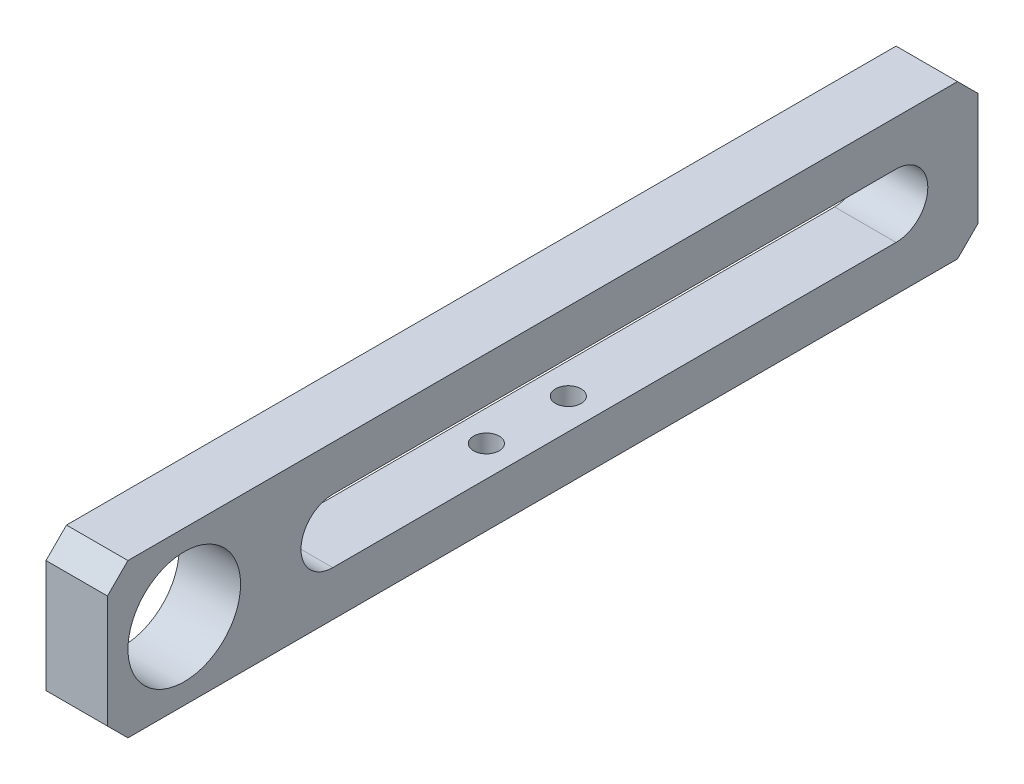
SolidWorks part; units mm, degrees
material "6061-T6"
ref_plane "Front Plane" through (0, 0, 0) normal (0, 0, 1) x (1, 0, 0)
ref_plane "Top Plane" through (0, 0, 0) normal (0, 1, 0) x (1, 0, 0)
ref_plane "Right Plane" through (0, 0, 0) normal (1, 0, 0) x (0, 0, -1)
sketch "Sketch1" plane through (0, 0, 0) normal (1, 0, 0) x (0, 0, -1)
  line L0 (22, -4.4) -> (77, -4.4)
  line L1 (0, 0) -> (85, 0)
  line L2 (0, 0) -> (0, -15)
  line L3 (0, -15) -> (85, -15)
  line L4 (85, 0) -> (85, -15)
  line L5 (22, -10.6) -> (77, -10.6)
  arc A0 (77, -10.6) -> (77, -4.4) centre (77, -7.5) ccw
  arc A1 (22, -4.4) -> (22, -10.6) centre (22, -7.5) ccw
  dimension "D6" = 6.2
  dimension "D1" = 85
  dimension "D2" = 15
  dimension "D3" = 8
  dimension "D4" = 7.5
  dimension "D5" = 55
extrude "Extrude1" add sketch "Sketch1" along normal blind 6
hole_wizard "M12x1.0 Tapped Hole1" positions "Sketch4" profile "Sketch3" tap size "M12x1.25" standard "ISO" end condition through all
sketch "Sketch4" plane through (6, 0, 0) normal (1, 0, 0) x (0, 0, -1)
  line L1 (0, -15) -> (85, -15) construction
  line L2 (0, 0) -> (0, -15) construction
  point P0 (7.5, -7.5)
  dimension "D1" = 7.5
  dimension "D2" = 7.5
sketch "Sketch3" plane through (6, -7.5, -7.5) normal (0, 1, 0) x (0, 0, -1)
  line L0 (0, 0) -> (0, 6)
  line L1 (0, 6) -> (5.5, 6)
  line L2 (5.5, 6) -> (5.5, 0)
  line L5 (5.5, 0) -> (0, 0)
  line L11 (0, -6.35) -> (0, 107.95) construction
  dimension "籵謂蹟恇謂郰芛眻噤" = 11
  dimension "籵謂蹟恇謂郰芛旮僅" = 6
cosmetic thread "Cosmetic thread1" parameters "D2"=12
chamfer "Chamfer1" distance 2 angle 45 4 edges at (3, 0, -85) (3, -15, -85) (3, -15, 0) (3, 0, 0)
hole_wizard "M3 Tapped Hole1" positions "Sketch9" profile "Sketch10" tap size "M3" standard "ISO"
sketch "Sketch9" plane through (0, -15, 0) normal (0, -1, 0) x (1, 0, 0)
  line L0 (0, 0) -> (6, 0) construction
  point P0 (3, -40)
  point P2 (3, -48)
  point P8 (3, 0)
  dimension "D1" = 8
  dimension "D2" = 40
sketch "Sketch10" plane through (3, -15, -40) normal (1, 0, 0) x (0, 0, -1)
  line L0 (0, 0) -> (0, 9.2511)
  line L1 (0, 9.2511) -> (1.25, 8.5)
  line L2 (1.25, 8.5) -> (1.25, 0)
  line L5 (1.25, 0) -> (0, 0)
  line L10 (0, 9.2511) -> (-1.25, 8.5) construction
  line L11 (0, -6.35) -> (0, 107.95) construction
  dimension "螺纹孔钻头直径" = 2.5
  dimension "螺纹孔钻头深度" = 8.5
  dimension "导头角度" = 118
cosmetic thread "Cosmetic thread2" parameters "D1"=4.75, "D2"=3
cosmetic thread "Cosmetic thread3" parameters "D1"=4.7596, "D2"=3
